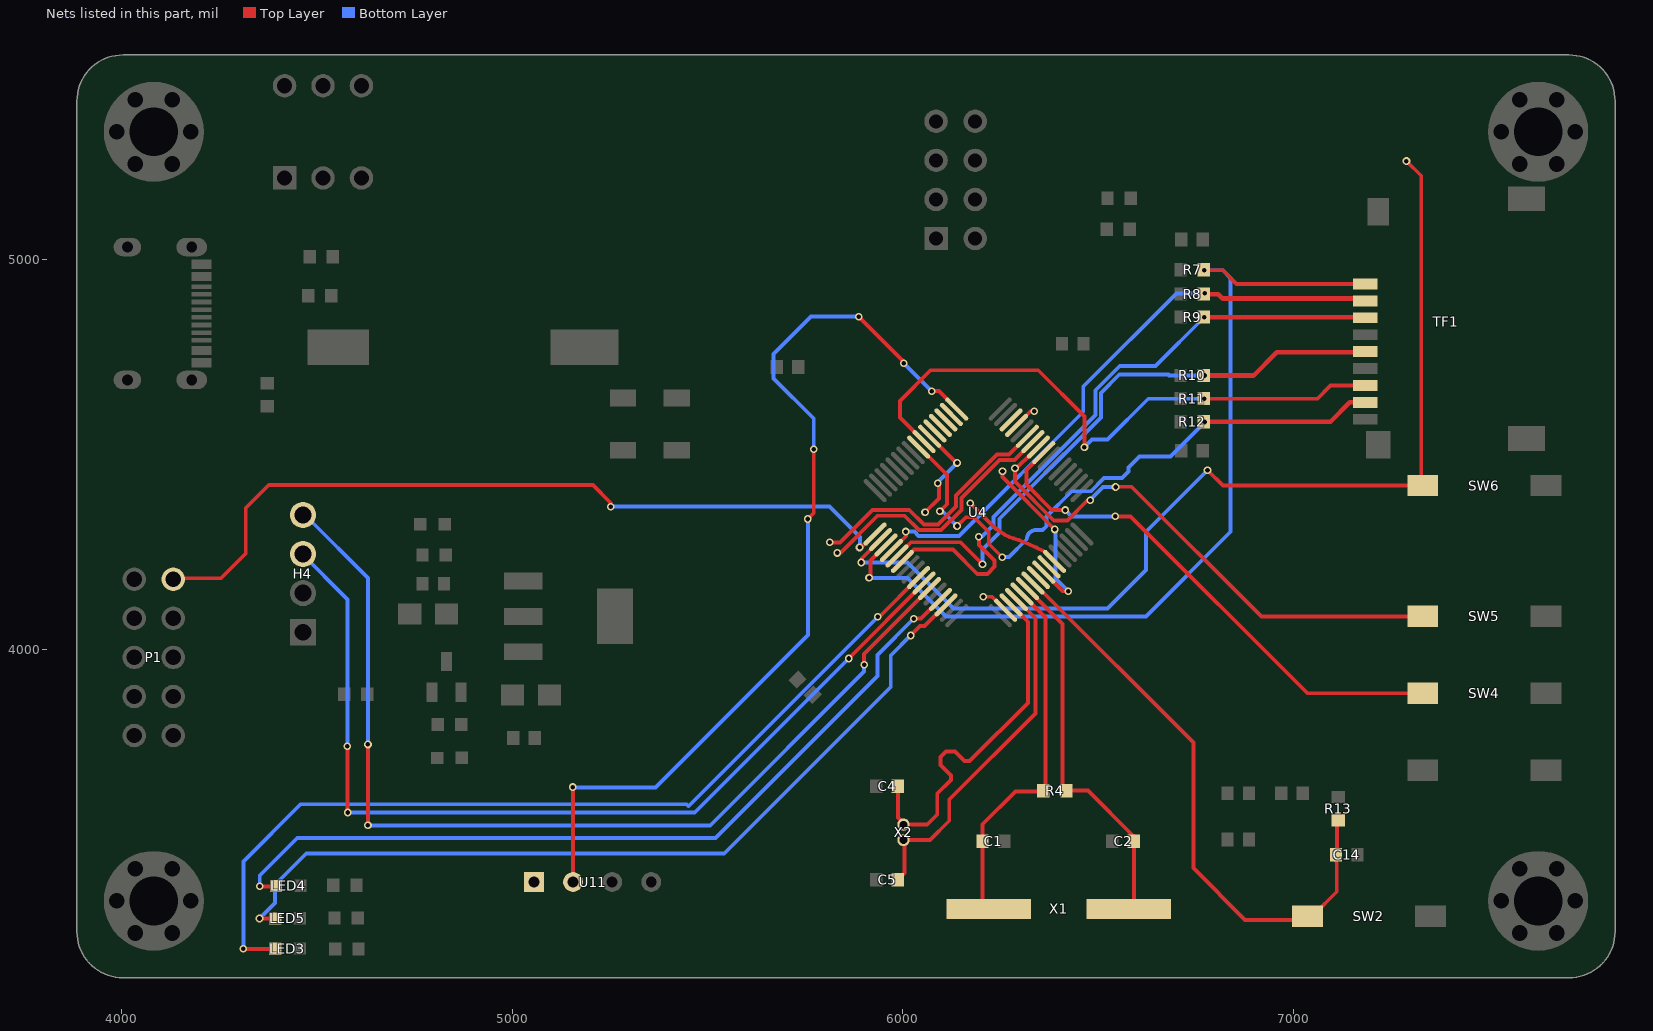
[diagram p0: the nets of this part, all layers, seen from the top]
# Altium PCB MISC52064.pcbdoc (part 2 of 2)
Units mil, origin at the board's own origin, x right, y up, seen from the top; angles counter-clockwise.
Board outline 3937.01 x 2362.2 mil, 2 copper layers (Top Layer, Bottom Layer), stack 62.205 mil thick; 65 components, 70 nets, 266 pads, 190 vias.

## Via types
v1: diameter 19.68, hole 11.8, Top Layer to Bottom Layer, 190 vias

## Nets (pads, with @x,y where several pads share a name; then routed paths per layer and width w, separated by ;. In a path a pad name is that pad's centre, name@x,y a point inside that pad or via, vN(x,y) a via of type N, cw(c..) or ccw(c..) an arc to the next point about the centre after c; other vN are vias at no path point) (continued)
PA14: P1.2 U4.49 | length 2063.8
  Top Layer w10: P1.2@4127.52,4174.39 P1.2@4136.38,4183.24 ; P1.2@4132.65,4183.24 P1.2@4136.38,4183.24 ; v1@5252.59,4366.08 5252.59,4376.32 5206.94,4421.96 4377.35,4421.96 4318.51,4363.12 4318.51,4246.24 4255.51,4183.24 P1.2@4136.38,4183.24 ; v1(5889.48,4262.14) 5893.35,4262.14 5917.12,4285.9 U4.49@5917.99,4285.9
  Bottom Layer w10: v1(5252.98,4366.56) 5812.97,4366.56 5890.24,4289.28 5890.24,4262.35 v1@5890.42,4262.17
PA15: SW6.1 U4.50 | length 2631.1
  Top Layer w10: v1(5894.12,4223.6) 5894.12,4233.11 U4.50@5943.3,4282.29 ; v1(6779.94,4459.82) 6819.31,4420.45 SW6.1@7326.99,4420.45 ; v1@7290,5250.46 7326.99,5213.48 SW6.1@7326.99,4420.45 ; SW6.1@7331.13,4420.45 SW6.1@7326.99,4420.45
  Bottom Layer w10: v1(5894.12,4223.6) 6012.23,4223.6 6130.34,4105.49 6524.04,4105.49 6622.46,4203.91 6622.46,4302.34 v1(6779.94,4459.82)
  other v1: 7289.17,5251
PB0: U4.26 | length 664.7
  Top Layer w10: v1@5842.02,4249.68 5935.67,4343.32 6004.73,4343.32 6041.71,4306.34 6098.35,4306.34 6150.4,4358.39 6150.4,4388.83 6247.51,4485.94 6286.11,4485.94 U4.26@6338.64,4538.47
  other v1: 5832.43,4248.14
PB1: U4.27 | length 624.9
  Top Layer w10: v1@5816.27,4275.1 5839.45,4275.1 5922.13,4357.79 6016.73,4357.79 6054.15,4320.36 6090.07,4320.36 6136.4,4366.69 6136.4,4394.63 6241.71,4499.94 6272.21,4499.94 U4.27@6292.33,4520.06
  other v1: 5812.96,4275.08
PB5: LED3.1 U4.57 | length 2339.1
  Top Layer w10: v1(4312.24,3234.81) 4393.16,3234.81 LED3.1@4393.71,3235.35 ; v1(5936.24,4084.81) 5940.68,4084.81 U4.57@6040.73,4184.86
  Bottom Layer w10: v1(4312.24,3234.81) 4312.24,3458.81 4458.24,3604.81 5446.24,3604.81 5451.24,3599.81 v1(5936.24,4084.81)
PB6: H4.3 U4.58 | length 2436.4
  Top Layer w10: v1@4578,3750.53 v1@4578.95,3749.57 ; v1(4578.39,3753.08) 4579.24,3752.22 v1(4579.24,3583.81) ; v1(5861.75,3978.03) U4.58@6054.65,4170.94
  Bottom Layer w10: H4.3@4457.84,4250.39 4578.92,4129.31 4578.92,3754.31 v1@4579.34,3753.89 ; v1(4579.24,3583.81) 5467.53,3583.81 v1(5861.75,3978.03)
PB7: H4.4 U4.59 | length 2571.2
  Top Layer w10: v1(4631.09,3550.81) v1(4631.09,3757.97) ; v1(5901.24,3961.81) 5901.24,3989.69 U4.59@6068.57,4157.02
  Bottom Layer w10: H4.4@4475.84,4339.51 4631.25,4184.1 v1@4631.25,3754.77 ; v1(4631.09,3550.81) 5507.24,3550.81 5901.24,3944.81 v1(5901.24,3961.81)
PB8: LED4.1 U4.61 | length 2136.3
  Top Layer w10: v1(4354.24,3394.81) 4394.9,3394.81 LED4.1@4395.77,3395.67 ; v1(6028.24,4079.81) 6047.04,4079.81 U4.61@6096.41,4129.18
  Bottom Layer w10: v1(4354.24,3394.81) 4354.24,3422.81 4450.24,3518.81 5521.24,3518.81 5935.24,3932.81 5935.24,3986.81 v1(6028.24,4079.81)
PB9: LED5.1 U4.62 | length 2204.3
  Top Layer w10: v1(4353.74,3312.31) 4354.11,3312.67 LED5.1@4393.77,3312.67 ; v1(6020.24,4036.81) 6044.24,4060.81 6055.88,4060.81 U4.62@6110.33,4115.26
  Bottom Layer w10: v1(4353.74,3312.31) 4393.24,3351.81 4393.24,3398.81 4473.24,3478.81 5543.24,3478.81 5969.24,3904.81 5969.24,3985.81 v1(6020.24,4036.81)
PB10: U4.29 | length 47.2
  Top Layer w10: U4.29@6300.4,4583.97 6327.04,4610.61 v1(6336.56,4610.61)
PB11: U4.30
PB12: U4.33 U11.2 | length 2384.2
  Top Layer w10: v1(5155.24,3648.81) 5156.24,3647.81 U11.2@5156.24,3405.81 ; v1(5757.24,4334.81) 5772.24,4349.81 v1(5772.24,4513.81) ; v1(5887.24,4852.81) 6002.24,4737.81 v1(6002.24,4733.81) ; v1(6073.96,4662.09) 6092.43,4662.09 U4.33@6138.17,4616.35
  Bottom Layer w10: v1(5155.24,3648.81) 5156.24,3647.81 5367.24,3647.81 5757.24,4037.81 v1(5757.24,4334.81) ; v1(5772.24,4513.81) 5772.24,4591.81 5669.24,4694.81 5669.24,4756.81 5765.24,4852.81 v1(5887.24,4852.81) ; v1(6002.24,4733.81) v1(6073.96,4662.09)
PB13: U4.34
PB14: U4.35
PB15: U4.36
PC0: U4.8
PC1: U4.9 | length 426.8
  Top Layer w10: v1@6255.06,4457.95 6255.06,4442.22 v1(6389.01,4308.27) ; U4.9@6381.78,4177.29 6408.83,4150.24 v1@6423.56,4150.24
  Bottom Layer w10: v1@6390.73,4305.14 6390.73,4182.97 v1(6423.56,4150.14)
  other v1: 6255.32,4457.36
PC2: U4.10
PC3: U4.11 | length 230.9
  Top Layer w10: v1(6172.4,4375.21) 6173.72,4375.21 6237.79,4311.14 ; 6238.98,4309.74 ccw(c6333.82,4428.03) 6297.26,4280.89 ; 6297.61,4280.54 cw(c6095.87,3734.98) U4.11@6364.69,4250.8
PC4: SW4.1 U4.24 | length 1336.7
  Top Layer w10: U4.24@6360.87,4505 6316.24,4460.37 6316.24,4422.81 6381.24,4357.81 v1(6416.24,4357.81) ; v1(6543.72,4341.71) 6583.09,4341.71 7035.85,3888.95 SW4.1@7331.13,3888.95
  Bottom Layer w10: v1(6416.24,4357.81) 6432.35,4341.71 v1(6543.72,4341.71)
PC5: SW5.1 U4.25 | length 1348.6
  Top Layer w10: U4.25@6329.14,4502.85 6291.44,4465.15 v1(6287.35,4465.15) 6287.14,4464.95 6287.14,4430.47 6386.57,4331.04 6421.22,4331.04 6473.2,4383.01 v1@6478.82,4383.01 ; v1@6544.41,4417.27 6544.69,4417.55 6585.99,4417.55 6917.74,4085.8 SW5.1@7331.13,4085.8
  Bottom Layer w10: v1@6480.26,4384.7 6512.5,4416.94 v1(6544.74,4416.94)
  other v1: 6479.61,4383.08
PC6: U4.37
PC7: U4.38 | length 234.5
  Top Layer w10: v1(6057.11,4352.2) 6092.56,4387.65 6092.56,4422.88 v1@6089.34,4426.1 ; U4.38@6087.32,4528.43 6137.34,4478.41 v1(6139.08,4478.41)
  Bottom Layer w10: v1(6089.79,4426.76) 6089.79,4429.12 v1(6139.08,4478.41)
PC8: R11.1 TF1.7 U4.39 | length 1546.4
  Top Layer w10: U4.39@6054.65,4532.83 5992.54,4594.95 5992.54,4636.98 6071.28,4715.72 6346.87,4715.72 6464.98,4597.61 v1(6464.98,4518.87) ; v1(6771.24,4642.81) 7061.36,4642.81 7095.27,4676.71 TF1.7@7183.43,4676.71
  Bottom Layer w10: v1(6464.98,4518.87) 6484.67,4538.56 6524.04,4538.56 6628.29,4642.81 v1(6771.24,4642.81)
PC9: R12.1 TF1.8 U4.40 | length 1550.3
  Top Layer w10: U4.40@6051.52,4509.63 6112.92,4448.23 6112.92,4372.67 v1@6097.24,4356.99 ; v1(6139.04,4316.97) 6161.44,4339.37 6182.51,4339.37 6220.17,4301.71 6220.17,4271.5 v1(6254.56,4237.11)
  Top Layer w11.8: R12.1@6770.23,4584.2 7094.83,4584.2 7144.03,4633.4 TF1.8@7183.43,4633.4
  Bottom Layer w10: v1(6095.15,4354.94) 6101.07,4354.94 v1(6139.04,4316.97) ; v1@6253.59,4238.1 6272.33,4238.1 6317.31,4283.08 cw(c6341.79,4282.44) 6342.4,4306.92 ; 6341.36,4306.98 6358.15,4306.98 6367.65,4316.48 6367.65,4341.19 6432.51,4406.06 6481.81,4406.06 6515.29,4439.54 6560.68,4439.54 6577.38,4456.23 6577.38,4466.7 6605.46,4494.78 6684.78,4494.78 v1(6773.2,4583.21)
PC10: R7.1 TF1.1 U4.51 | length 2311.5
  Top Layer w10: v1(5913.8,4184.23) 5917.65,4188.07 5917.65,4228.81 U4.51@5957.22,4268.38 ; R7.1@6770.23,4972.74 6771.34,4971.63 6819.31,4971.63 6854.39,4936.55 TF1.1@7183.43,4936.55
  Bottom Layer w10: v1(5913.8,4184.23) 6012.23,4184.23 6110.65,4085.8 6622.46,4085.8 6839,4302.34 6839,4951.94 6819.31,4971.63 v1(6771.24,4971.63)
PC11: R8.1 TF1.2 U4.52 | length 1518.6
  Top Layer w10: U4.52@5992.76,4275.64 6007.86,4290.74 v1(6007.86,4302.71)
  Top Layer w11.8: R8.1@6770.23,4910.63 6807.85,4910.63 6819.31,4899.16 7177.53,4899.16 TF1.2@7183.43,4893.25
  Bottom Layer w10: v1(6007.86,4302.71) 6029.58,4302.71 6040.79,4291.49 6144.2,4291.49 6462.08,4609.37 6462.08,4674.12 6700.23,4912.27 v1(6773.01,4912.27)
PC12: R10.1 TF1.5 U4.53 | length 1514.6
  Top Layer w10: U4.53@6007.34,4261.15 6021.62,4275.44 6148.2,4275.44 v1@6204.83,4218.81
  Top Layer w11.8: R10.1@6770.23,4702.31 6898.05,4702.31 6957.11,4761.36 7181.46,4761.36 TF1.5@7183.43,4763.33
  Bottom Layer w10: v1(6203.99,4219.44) 6203.99,4256.55 6203.88,4256.66 6247.63,4300.42 6247.63,4335.53 6507.02,4594.92 6507.02,4657.43 6554.19,4704.6 6679.65,4704.6 6681.96,4702.29 v1(6772.18,4702.29)
PC13: U4.2 | length 45.1
  Top Layer w10: v1(6205.96,4135.91) 6228.94,4135.91 U4.2@6244.55,4120.3
PC14: C4.2 U4.3 X2.1 | length 915.5
  Top Layer w10: C4.2@5987.32,3651.05 5987.32,3570.42 X2.1@6003.36,3554.39 ; X2.1@6001.74,3552.77 X2.1@6004.98,3552.77 ; X2.1@6005.27,3552.48 X2.1@6004.98,3552.77 ; U4.3@6297.08,4095.24 6320.46,4071.86 6320.46,3864.49 6171.33,3715.36 6158.22,3715.36 6133.91,3739.67 6110.47,3739.67 6096.6,3725.81 6096.6,3705.2 6123,3678.8 6123,3667.23 6088.37,3632.6 6088.37,3578.49 6062.65,3552.77 X2.1@6004.98,3552.77
PC15: C5.2 U4.4 X2.2 | length 922.6
  Top Layer w10: C5.2@5987.32,3411.66 6004.13,3428.48 X2.2@6004.13,3511.07 ; X2.2@6001.74,3513.4 X2.2@6006.55,3513.4 ; X2.2@6006.16,3513.01 X2.2@6006.55,3513.4 ; U4.4@6291.27,4129.18 6339.64,4080.82 6339.64,3837.42 6119.07,3616.84 6119.07,3562.68 6069.79,3513.4 X2.2@6006.55,3513.4
PD0: C1.2 R4.2 U4.5 X1.2 | length 939.2
  Top Layer w10: X1.2@6205.75,3332.46 6204.34,3333.87 C1.2@6204.34,3510.27 6204.34,3553.66 6288.56,3637.87 R4.2@6357.18,3637.87 ; U4.5@6305.19,4143.1 6365.77,4082.52 6365.77,3652.59 R4.2@6355.77,3642.59
PD1: C2.2 R4.1 U4.6 X1.1 | length 943.4
  Top Layer w10: U4.6@6334.89,4140.92 6409.17,4066.64 6409.17,3649.48 R4.1@6419.17,3639.48 6420.1,3640.4 6473.62,3640.4 C2.2@6589.96,3524.07 ; X1.1@6588.57,3337.57 6591.39,3340.38 C2.2@6591.39,3510.06 C2.2@6591.39,3524.07
PD2: R9.1 TF1.3 U4.54 | length 1670.2
  Top Layer w10: U4.54@5980.15,4208.04 6028.65,4256.54 6128.79,4256.54 6190.72,4194.61 6216.45,4194.61 6234.97,4213.12 6234.97,4228.5 6195.01,4268.45 v1@6195.01,4285.85
  Top Layer w11.8: R9.1@6770.23,4851.71 7181.66,4851.71 TF1.3@7183.43,4849.94
  Bottom Layer w10: v1@6194.86,4289.71 6202.39,4289.71 6232.57,4319.88 6232.57,4340.26 6493.02,4600.72 6493.02,4664.44 6555.48,4726.89 6647.29,4726.89 v1(6771.69,4851.3)
  other v1: 6194.42,4289.28
RESET: C14.2 R13.1 SW2.1 U4.7 | length 1440.5
  Top Layer w10: U4.7@6349.12,4157.64 6743.85,3762.91 6743.85,3441.25 6876.34,3308.77 SW2.1@7018.41,3308.77 ; SW2.1@7051.52,3322.4 7052.37,3322.4 7110.85,3380.88 7110.85,3458.2 C14.2@7109.31,3459.74 ; 7111.45,3493.61 R13.1@7111.45,3561.69
VCC: U11.1
pads on no net: P1.3 P1.9 SW1.1 SW1.4 SW1.5 SW1.6 TF1.9 U3.4 U6.2 U6.3 U6.6 U6.7 U11.3 USB1.1 USB1.2 USB1.3 USB1.4 USB1.A5 USB1.A8 USB1.B5 USB1.B8

## Polygon pours and split planes (outlines as drawn)
GND on Top Layer (solid, remove dead copper, pour order 2): 3712.18,5550.74 3712.18,3081.04 7994.47,3081.04 7994.47,5550.74
D+ on Top Layer (solid, remove dead copper, pour order 0): 4318.39,4870.68 4377.55,4870.68 4377.55,4779.4 4372.67,4774.53 4372.67,4779.76 4321.06,4831.37 4318.04,4831.37
GND on Bottom Layer (solid, remove dead copper, pour order 6): 3000,5646.93 3000,3000 7916.52,3000 7916.52,5646.93
5VOUT on Bottom Layer (solid, remove dead copper, pour order 4): 3787.66,3711.22 4284.49,3710.25 4283.63,3802.1 4346.9,3791.09 4426.63,3712.07 4868.15,3711.22 4878.86,3721.92 4960.59,3721.92 4968.88,3713.64 4968.88,3467.83 4930.81,3429.77 4735.49,3430.01 4734.63,3157.35 3787.66,3159.44

## Keep-outs
Top Layer:
  region: 4194.04,5050.95 4195.8,5052.71 4195.8,5004 4178.79,4986.99 4178.79,4938.21 4182.57,4934.43 4155.12,4906.98 4155.12,4790.3 4151.6,4786.78 4151.6,4785.9 4174.48,4763.01 4174.48,4669.71 4173.6,4668.83 4001.08,4668.83 3994.03,4675.87 3994.03,5035.01 4009.98,5050.95
  region: 6188.18,4715.09 6517.51,4385.77 6517.51,4321.19 6488.77,4292.46 6488.77,4264.37 6490.47,4262.67 6282.9,4055.1 6260.78,4055.1 6207.91,4107.97 6170.73,4107.97 5947.02,4331.68 5947.02,4374.28 5885.39,4435.91 6164.57,4715.09
Board Outline Layer:
  the board outline again, w10

## Other copper
Top Layer:
  region net PD2: 6032.19,4253 6025.12,4260.08 6018.46,4254.45 6026.82,4246.1
  region net PC11: 6004.32,4294.28 5990.63,4282.29 5998.98,4273.94 6010.99,4286.81
  region net GND: 5903.63,4453.36 5915.46,4440.97 5923.81,4449.32 5909.5,4461.64
  region net PA13: 5924.67,4475.31 5917.12,4468.73 5929.38,4454.88 5937.73,4463.23
  region net PA10: 6039.13,4443.43 6026.82,4457.67 6018.46,4449.32 6030.98,4437.43
  region net PA9: 5972.73,4524.94 5985.05,4510.56 5993.41,4518.91 5981.11,4530.7
  region net PC7: 6102.05,4506.63 6108.43,4514.39 6096.41,4527.26 6088.06,4518.91
  region net GND: 6238.01,4569.5 6243.95,4574.59 6235.6,4582.94 6230.93,4576.57
  region net PB10: 6330.58,4607.08 6323.51,4614.15 6310.76,4602.43 6319.11,4594.08
  region net BOOT1: 6336.56,4584.97 6329.49,4592.04 6326.4,4589.71 6334.21,4581.86
  region net PB0: 6293.01,4499.91 6300.04,4492.8 6313.54,4505 6305.19,4513.35
  region net 3.3V: 6398.46,4395.67 6410.98,4407.56 6402.63,4415.91 6390.32,4401.67
  region net GND: 6477.48,4461.54 6463.87,4449.32 6472.22,4440.97 6484.38,4454.29
  region net PA1: 6484.56,4247.94 6472.22,4262.81 6463.87,4254.45 6474.83,4243.52
  region net PA0: 6470.56,4235.12 6458.31,4248.89 6449.95,4240.54 6463.1,4228.43
  region net $1N7223: 6450.19,4214.31 6456.32,4222.33 6444.38,4234.97 6436.03,4226.61
  region net GND: 6442.56,4207.95 6430.47,4221.05 6422.12,4212.7 6435.92,4200.44
  region net PC1: 6401.01,4165.13 6388.71,4179.29 6380.35,4170.94 6392.99,4159
  region net PD1: 6359.22,4123.67 6346.95,4137.53 6338.6,4129.18 6351.63,4117.11
  region net PD0: 6345.22,4110.14 6333.03,4123.61 6324.68,4115.26 6338.15,4103.07
  region net PC15: 6324.23,4089.16 6331.3,4096.23 6319.11,4109.7 6310.76,4101.34
  region net PC14: 6317.45,4081.94 6305.19,4095.77 6296.84,4087.42 6309.91,4075.34
  region net PC13: 6225.4,4132.38 6235.6,4120.83 6243.95,4129.18 6232.48,4139.45
  region net $1N6590: 6282.78,4047.33 6289.45,4054.8 6277.35,4067.93 6269,4059.58
  region net PD1: 6596.39,3377.6 6586.39,3377.6 6573.89,3362.6 6608.89,3362.6
  region net PD0: 6209.34,3377.6 6199.34,3377.6 6186.84,3362.6 6221.84,3362.6
  region net 3.3V: 4949.95,4082.19 4979.95,4064.15 4979.95,4107.45 4949.95,4102.19
  region net 3.3V: 4431.36,4145.86 4421.91,4107.34 4429.28,4100.56 4468.31,4111.88
  region net 3.3V: 4488.06,4121.08 4507.07,4141.66 4507.07,4151.66 4485.81,4171.23
  region net 3.3V: 5450.4,4601.99 5476.35,4604.32 5455.14,4660.89 5388.21,4623.2
  region net $1N6590: 5427,4474.34 5439.5,4489.34 5404.5,4489.34 5417,4474.34
  region net $1N6590: 5358.21,4522.11 5358.21,4502.11 5388.21,4489.34 5388.21,4532.65
  region net $1N4980: 5242.08,4687.72 5229.2,4672.32 5250.42,4623.2 5250.42,4666.51
  region net $1N6590: 5347.35,4522.11 5317.35,4532.65 5317.35,4489.34 5347.35,4502.11
  region net $1N7223: 6881.24,3547.65 6870.5,3532.65 6901.99,3532.65 6891.24,3547.65
  region net 3.3V: 6414.69,4756.89 6423.39,4765.64 6392.19,4765.64 6404.69,4756.89
  region net 3.3V: 5804.61,3889.99 5777.11,3902.49 5774.33,3867.49 5801.83,3879.99
  region net 3.3V: 5742.58,4688.12 5748.34,4706.12 5716.85,4706.12 5730.58,4688.12
  region net GND: 5655.17,4695.51 5661.73,4706.12 5661.73,4741.55 5651.12,4705.6
  region net PC14: 5992.32,3618.33 6003.07,3633.33 5971.57,3633.33 5982.32,3618.33
  region net PC15: 6000.6,3432.01 5980.29,3429.38 6003.07,3402.66 6007.67,3424.94
  region net PD0: 6209.34,3477.56 6220.09,3492.56 6188.6,3492.56 6199.34,3477.56
  region net PD0: 6199.34,3542.99 6188.6,3527.99 6220.09,3527.99 6209.34,3542.99
  region net PD1: 6596.39,3477.34 6607.14,3492.34 6575.64,3492.34 6586.39,3477.34
  region net PD1: 6568.57,3538.38 6575.64,3513.64 6607.14,3527.78 6582.71,3538.38
  region net PD0: 6328.97,3642.87 6328.97,3632.87 6343.97,3622.47 6343.97,3655.37
  region net PD0: 6370.77,3671.49 6360.77,3671.49 6348.27,3656.49 6375.73,3656.49
  region net PD1: 6414.17,3671.49 6404.17,3671.49 6403.29,3656.49 6426.67,3656.49
  region net PD1: 6450.05,3635.4 6450.05,3645.4 6435.05,3656.49 6435.05,3622.9
  region net $1N7223: 6883.22,3665.76 6870.72,3650.76 6901.99,3650.76 6893.22,3665.76
  region net $1N7223: 6916.99,3628.05 6916.99,3638.05 6901.99,3650.55 6901.99,3615.55
  region net $1N7223: 6881.24,3600.33 6891.24,3600.33 6901.99,3615.33 6870.5,3615.33
  region net 3.3V: 7054.78,3628.05 7054.78,3638.05 7039.78,3650.05 7039.78,3616.04
  region net $1N7223: 6938.18,3628.05 6953.18,3616.04 6953.18,3650.05 6938.18,3638.05
  region net D-: 4246.28,4884.82 4246.28,4894.82 4231.28,4896.34 4231.28,4884.53
  region net D+: 4246.28,4875.68 4231.28,4876.65 4231.28,4864.84 4246.28,4865.68
  region net D+: 4246.28,4836.37 4231.28,4837.28 4231.28,4825.47 4246.28,4826.37
  region net 5VOUT: 4993.79,3726.71 5013.79,3726.71 5018.75,3756.71 4987.25,3756.71
  region net 5VOUT: 5011.64,3822.15 4991.64,3822.15 4987.25,3792.15 5018.75,3792.15
  region net 3.3V: 4840.14,4216.91 4820.14,4216.91 4810.1,4186.91 4841.6,4186.91
  region net 3.3V: 6705.91,4734.32 6695.04,4719.32 6726.79,4719.32 6715.91,4734.32
  region net 3.3V: 6705.91,4670.3 6715.91,4670.3 6726.79,4685.3 6695.04,4685.3
  region net PC12: 6803.81,4708.21 6786.11,4719.32 6786.11,4685.3 6803.81,4696.41
  region net 3.3V: 6705.91,4611.25 6715.91,4611.25 6726.79,4626.25 6695.04,4626.25
  region net 3.3V: 6705.91,4675.26 6695.04,4660.26 6726.79,4660.26 6715.91,4675.26
  region net 3.3V: 6680.04,4584.75 6680.04,4574.75 6695.04,4567.19 6695.04,4597.25
  region net 3.3V: 6705.91,4616.21 6695.04,4601.21 6726.79,4601.21 6715.91,4616.21
  region net PC9: 6803.81,4590.1 6786.11,4601.21 6786.11,4567.19 6803.81,4578.3
  region net 3.3V: 6705.91,4819.7 6715.91,4819.7 6726.79,4834.7 6695.04,4834.7
  region net PD2: 6803.81,4857.61 6786.11,4868.72 6786.11,4834.7 6803.81,4845.81
  region net 3.3V: 7146.6,3628.34 7131.6,3639.21 7131.6,3607.46 7146.6,3618.34
  region net 3.3V: 7082.58,3628.05 7097.58,3615.55 7097.58,3639.21 7082.58,3638.05
  region net $1N170341: 4873.81,3840.73 4863.81,3840.73 4853.64,3825.73 4885.39,3825.73
  region net $1N170394: 4812.27,3776.71 4824.77,3791.71 4794.32,3791.71 4802.27,3776.71
  region net $1N170394: 4812.27,3754.21 4802.27,3754.21 4792.8,3739.21 4824.29,3739.21
  region net $1N4980: 5229.68,4699.5 5254.68,4729.5 5184.68,4729.5 5209.68,4699.5
  region net PA14: 4154.77,4159.96 4184.49,4178.24 4183.64,4188.24 4150.96,4204.8
  region net PA13: 4155.33,4060.56 4184.6,4079.06 4183.48,4089.06 4150.3,4105.28
  region net 3.3V: 4062.48,3874.65 4075.1,3909.69 4069.03,3917.77 4035.43,3910.61
  region net PA9: 4155.85,3861.16 4184.71,3879.84 4183.31,3889.84 4149.64,3905.72
  region net PA10: 4146.24,3753.74 4182.42,3767.73 4185.18,3777.73 4158.21,3797.12
  region net 3.3V: 4840.14,4195.61 4846.02,4225.61 4814.27,4225.61 4820.14,4195.61
  region net 3.3V: 4876.02,4253.28 4846.02,4259.62 4846.02,4225.61 4876.02,4233.28
  region net $1N123092: 4760.82,4289.62 4754.95,4259.62 4786.7,4259.62 4780.82,4289.62
  region net BOOT1: 6593.9,5044.32 6597.17,5059.32 6571.4,5059.32 6583.9,5044.32
  region net 5VOUT: 4991.64,3941.17 4972.11,3911.17 5031.16,3911.17 5011.64,3941.17
  region net 5VOUT: 5011.64,3827.67 5031.16,3857.67 4972.11,3857.67 4991.64,3827.67
  region net 3.3V: 4827.74,4050.44 4837.74,4050.44 4850.24,4065.44 4815.24,4065.44
  region net 3.3V: 4892.1,4082.19 4892.1,4102.19 4862.1,4118.94 4862.1,4065.44
  region net 3.3V: 4822.58,4148.94 4803.05,4118.94 4862.1,4118.94 4842.58,4148.94
  region net BOOT0: 6497.46,5147.09 6497.46,5132.95 6521.37,5139.17 6508.07,5173.19
  region net PA0: 7276.76,3700.6 7276.76,3690.6 7291.76,3678.1 7291.76,3713.1
  region net 3.3V: 7601.24,3654.33 7615.38,3654.33 7643.67,3664.93 7606.72,3677.48
  region net PC5: 7276.76,4090.8 7276.76,4080.8 7291.76,4068.3 7291.76,4103.3
  region net PC11: 7134.23,4893.26 7151.93,4879.45 7151.93,4907.05 7134.23,4905.06
  region net PD2: 7134.23,4857.61 7134.23,4845.81 7151.93,4836.14 7151.93,4863.74
  region net 3.3V: 7136.93,4801.63 7151.93,4792.83 7151.93,4820.43 7136.93,4811.63
  region net PC12: 7134.23,4767.26 7134.23,4755.46 7151.93,4749.53 7151.93,4777.13
  region net PC9: 7144.03,4639.3 7144.03,4627.5 7151.93,4619.6 7151.93,4647.2
  region net PC11: 6803.81,4904.73 6803.81,4916.53 6786.11,4927.64 6786.11,4893.62
  region net PC14: 6012.15,3540.96 6028.51,3547.77 6028.51,3557.77 6012.15,3564.58
  region net PC14: 6005,3568.18 5990.86,3573.96 5983.78,3566.89 5986.04,3554.08
  region net PC15: 5991.65,3501.31 5999.13,3485.91 6009.13,3487.45 6015,3504.9
  region net PC15: 6012.15,3501.59 6028.51,3508.4 6028.51,3518.4 6012.15,3525.21
  region net 5V: 4494.1,5187.53 4506.82,5156.64 4526.82,5157.07 4539.09,5188.5
  region net $1N175343: 4763.03,3892.52 4763.03,3880.52 4781.03,3866.95 4781.03,3907.52
  region net $1N170341: 4873.81,3851.95 4883.38,3866.95 4855.83,3866.95 4863.81,3851.95
  region net 3.3V: 4803.43,3994 4803.43,3984 4818.43,3971.5 4818.43,3994.9
  region net 3.3V: 4827.74,4009.9 4818.43,3994.9 4845.98,3994.9 4837.74,4009.9
  region net D+: 4451.7,4880.59 4478.36,4889.57 4462.31,4923.01 4451.7,4894.73
  region net D-: 4450.99,4996.96 4465.99,4988.89 4465.99,5019.46 4450.99,5006.96
  region net 3.3V: 4400.92,4597.79 4390.32,4626.08 4356.3,4607.41 4387.77,4596.8
  region net D+: 4367.67,4713.48 4356.3,4698.48 4390.17,4698.48 4377.67,4713.48
  region net $1N175343: 4663.5,3892.52 4645.5,3903.52 4645.5,3869.51 4663.5,3880.52
  region net PA9: 4536.43,3890.84 4536.43,3878.84 4554.43,3869.51 4554.43,3903.52
  region net PC13: 6212.47,4128.53 6222.7,4130.91 6222.7,4140.91 6212.47,4143.29
  region net 3.3V: 6402.3,4777.5 6404.69,4767.27 6414.69,4767.27 6417.07,4777.5
  region net 3.3V: 5729.2,4717.91 5730.58,4707.68 5742.58,4707.68 5743.96,4717.91
  region net PC11: 6000.48,4296.2 6002.86,4290.74 6012.86,4290.74 6015.24,4296.2
  region net PC5: 6296.56,4461.68 6303.59,4470.23 6298.69,4479.48 6289.64,4474.72
  region net PC5: 6279.83,4458.8 6282.14,4448.52 6292.14,4448.32 6294.59,4458.49
  region net PC9: 6104.98,4354.3 6110.53,4363.21 6103.48,4370.3 6094.56,4364.77
  region net 3.3V: 6696.2,4587.47 6686.23,4584.75 6687.43,4574.75 6697.95,4572.81
  region net 3.3V: 6395.34,4389.72 6401.34,4398.55 6395,4406.36 6386.03,4401.18
  region net PC7: 6066.94,4351.59 6072.48,4360.5 6065.41,4367.57 6056.5,4362.03
  region net PC7: 6138.46,4488.23 6129.48,4493.34 6123.31,4485.37 6129.41,4476.57
  region net PC7: 6084.54,4418.44 6087.56,4408.67 6097.56,4411.6 6098.71,4422.59
  region net BOOT1: 6596.29,4860.3 6593.9,4870.52 6583.9,4870.51 6581.52,4860.28
  region net BOOT1: 6368.11,4593.53 6356.59,4593.5 6351.42,4583.5 6361.33,4580.42
  region net BOOT0: 6591.19,4758.43 6582.29,4764.03 6575.12,4757.06 6580.61,4748.14
  region net BOOT0: 6133.99,4204.2 6128.76,4194.77 6140.7,4192.57 6148.51,4201.53
  region net PA0: 6553.09,4589.42 6562.01,4583.87 6569.08,4590.94 6563.53,4599.86
  region net PA1: 6532.51,4568.53 6541.42,4562.98 6548.49,4570.05 6542.95,4578.97
  region net PA1: 6549.62,4237.05 6539.37,4234.71 6539.23,4224.71 6549.43,4222.29
  region net PA1: 6610.6,4456.45 6601.69,4461.99 6594.62,4454.92 6600.16,4446.01
  region net PA0: 6527.88,4164.71 6535.72,4155.82 6547.57,4158.1 6542.38,4167.51
  region net PA0: 6528.9,4180.99 6519.49,4186.18 6517.21,4174.32 6526.11,4166.49
  region net PA0: 6654.73,4449.64 6645.81,4455.16 6638.79,4448.03 6644.37,4439.13
  region net PC12: 6778.71,4694.92 6788.93,4696.41 6788.91,4708.21 6778.68,4709.69
  region net PC9: 6780.42,4576.52 6790.51,4578.3 6789.32,4590.1 6778.93,4591.21
  region net PD2: 6778.5,4844.2 6788.67,4845.81 6788.17,4857.61 6777.89,4858.95
  region net PC11: 6778.2,4903.9 6788.7,4904.73 6790.7,4916.53 6780.65,4918.46
  region net PC5: 6551.69,4409.98 6561.77,4412.55 6561.15,4422.55 6550.78,4424.71
  region net PC5: 6471.15,4388.11 6463.05,4379.94 6466.49,4369.24 6475.68,4374.06
  region net PC3: 6172.72,4365.37 6181.68,4360.17 6188.08,4367.92 6182.12,4376.75
  region net 3.3V: 5860.23,4574.85 5862.61,4564.62 5872.61,4564.62 5874.99,4574.85
  region net $1N6590: 5374.26,4322.57 5379.74,4331.49 5372.55,4338.45 5363.65,4332.84
  region net $1N6590: 5473.94,4108.22 5482.85,4102.68 5489.92,4109.75 5484.38,4118.66
  region net PB0: 5840.08,4241.95 5849.13,4249.71 5847.09,4261.81 5837.62,4256.51
  region net PB0: 5840.08,4241.95 5849.13,4249.71 5847.09,4261.81 5837.62,4256.51
  region net PB1: 5819.49,4267.71 5829.7,4270.1 5829.68,4280.1 5819.45,4282.48
  region net PA14: 5260.05,4373.4 5252.69,4383.29 5239.18,4382.66 5245.3,4372.71
  region net PA14: 5260.05,4373.4 5252.69,4383.29 5239.18,4382.66 5245.3,4372.71
  region net PA14: 5898.74,4258.81 5905.68,4267.4 5900.66,4276.52 5891.62,4271.74
  region net PA13: 5293.95,4394.79 5296.39,4384.61 5306.39,4384.79 5308.71,4395.06
  region net PA13: 5718.12,4413.74 5715.74,4423.96 5705.74,4423.96 5703.36,4413.74
  region net PA9: 5967.35,4535.64 5969.74,4530 5979.74,4530 5982.12,4535.64
  region net PA10: 6042.86,4442.3 6034.08,4448.48 6026.01,4442.4 6031.07,4433.42
  region net PA9: 5824.44,4715.77 5814.22,4713.39 5814.22,4703.39 5824.44,4701
  region net PA10: 5831.83,4682.43 5821.61,4680.05 5821.61,4670.05 5831.83,4667.67
  region net PA9: 5692.09,4548.91 5689.45,4558.94 5679.45,4558.09 5677.38,4547.65
  region net PA9: 4376.23,3892.22 4366.01,3889.84 4366.01,3879.84 4376.23,3877.46
  region net PA9: 4389.25,3877.46 4399.47,3878.84 4399.47,3890.84 4389.25,3892.22
  region net PA10: 5681.2,4489.85 5686.71,4498.77 5679.58,4505.78 5670.67,4500.2
  region net PA10: 4418.72,3780.11 4408.5,3777.73 4408.5,3767.73 4418.72,3765.34
  region net PC12: 6204.76,4229.25 6195.85,4234.86 6188.68,4227.89 6194.16,4218.97
  region net PD2: 6187.44,4282.34 6190.01,4272.25 6200.01,4272.86 6202.18,4283.23
  region net PA15: 7288.76,5241.17 7297.69,5235.71 7304.61,5242.93 7298.97,5251.83
  region net PB10: 6329.81,4617.77 6319.82,4610.46 6320.27,4596.77 6330.29,4603.02
  region net PB10: 6329.81,4617.77 6319.82,4610.46 6320.27,4596.77 6330.29,4603.02
  region net PC9: 6148.86,4316.35 6154.4,4325.26 6147.33,4332.34 6138.42,4326.79
  region net PC9: 6255.17,4246.94 6246.26,4252.48 6239.19,4245.41 6244.73,4236.5
  region net PC1: 6417.13,4157.58 6408.83,4155.24 6408.83,4145.24 6416.98,4142.82
  region net PC1: 6247.77,4451.04 6250.06,4442.22 6260.06,4442.22 6262.53,4450.66
  region net GND: 6740.97,3853.9 6738.59,3864.12 6728.59,3864.12 6726.21,3853.9
  region net GND: 6193.84,4648.84 6201.8,4644.14 6208.88,4651.21 6204.53,4659.03
  region net GND: 5544.38,4677.38 5554.59,4679.78 5554.55,4689.78 5544.32,4692.14
  region net GND: 6497.51,4479.6 6488,4472.05 6489.3,4459.21 6498.99,4464.91
  region net GND: 6497.51,4479.6 6488,4472.05 6489.3,4459.21 6498.99,4464.91
Bottom Layer:
  region net PB6: 4461.49,4211.87 4500.5,4200.66 4507.83,4207.47 4498.27,4246.02
  region net PB7: 4466.53,4311.74 4504.55,4303.73 4510.82,4311.6 4497.77,4351.03
  region net 3.3V: 5732.19,4715.61 5740.54,4707.97 5750.6,4712.05 5745.87,4721.16
  region net PC11: 6014.37,4295.32 6024.59,4297.71 6024.59,4307.71 6014.37,4310.09
  region net PC9: 6098.77,4345.79 6107.91,4341.02 6111.67,4351.41 6103.79,4359.67
  region net 3.3V: 6697.02,4588.29 6686.8,4585.9 6686.82,4575.9 6697.04,4573.53
  region net 3.3V: 6257.27,4626.68 6256.84,4637.27 6244.84,4640.06 6242.89,4630.02
  region net 3.3V: 6395.47,4391.08 6400.88,4400.01 6393.56,4406.84 6384.67,4401.15
  region net PC7: 6129.26,4479.03 6123.72,4470.12 6130.79,4463.04 6139.7,4468.59
  region net PC7: 6099.58,4427.82 6104.56,4436.82 6096.27,4442.67 6087.52,4436.34
  region net BOOT1: 6579.14,4854.91 6573.37,4846.04 6580.07,4838.6 6589.01,4843.94
  region net BOOT1: 6378.25,4590.06 6376.07,4600.42 6366.07,4601 6363.51,4590.9
  region net BOOT0: 6583.93,4756 6573.71,4753.62 6573.71,4743.62 6583.93,4741.24
  region net BOOT0: 6152.12,4207.56 6158.16,4216.38 6151.88,4224.24 6142.91,4219.1
  region net PA0: 6588.89,4667.61 6591.27,4657.39 6601.27,4657.39 6603.65,4667.61
  region net PA1: 6553.83,4671.85 6556.22,4661.63 6566.22,4661.63 6568.6,4671.85
  region net PA0: 6560.92,4605.94 6558.46,4609.1 6548.46,4609.1 6546.16,4605.56
  region net PA1: 6538.44,4586.64 6535.42,4596.41 6525.42,4593.55 6524.24,4582.58
  region net PA1: 6565.86,4228.97 6571.4,4237.88 6564.33,4244.95 6555.42,4239.4
  region net PA1: 6603.47,4454.01 6593.94,4451.62 6593.94,4441.62 6603.47,4439.24
  region net PA0: 6543.72,4171.96 6549.24,4180.88 6542.12,4187.9 6533.21,4182.32
  region net PA0: 6644.37,4440.48 6638.8,4431.57 6645.84,4424.46 6654.76,4429.99
  region net PC12: 6765.67,4709.67 6755.45,4707.29 6755.45,4697.29 6765.67,4694.91
  region net PC9: 6763.38,4583.82 6757.83,4574.91 6764.9,4567.84 6773.81,4573.38
  region net PD2: 6761.87,4851.92 6756.32,4843 6763.39,4835.93 6772.31,4841.48
  region net PC11: 6766.5,4919.65 6756.27,4917.27 6756.27,4907.27 6766.5,4904.88
  region net PC5: 6538.23,4424.32 6528,4421.94 6528,4411.94 6538.23,4409.56
  region net 3.3V: 5872.82,4589.71 5864.7,4597.95 5853.81,4594.7 5858.68,4585.48
  region net $1N6590: 5357.04,4316.52 5359.43,4306.29 5369.43,4306.29 5371.81,4316.52
  region net $1N6590: 5475.93,4127.79 5467.08,4133.67 5459.46,4127.15 5464.72,4118.19
  region net PA14: 5259.49,4359.17 5269.71,4361.56 5269.71,4371.56 5259.49,4373.94
  region net PA14: 5897.34,4268.05 5895.24,4278.47 5885.24,4279.25 5882.63,4269.2
  region net PA13: 5309.99,4396.98 5319.76,4400.08 5315.78,4410.08 5304.53,4410.7
  region net PA13: 5702.77,4413.01 5692.95,4410.08 5695.19,4400.08 5706,4398.6
  region net PA9: 5975.35,4551.97 5966.44,4557.51 5959.37,4550.44 5964.91,4541.53
  region net PA10: 6041.5,4442.48 6032.59,4448.03 6025.52,4440.96 6031.06,4432.04
  region net PA9: 5837.79,4701.31 5847.91,4703.83 5847.45,4713.83 5837.12,4716.05
  region net PA10: 5843.88,4666.91 5854.42,4668.82 5854.96,4678.82 5845.73,4681.56
  region net PA9: 5675.47,4542.41 5669.93,4533.5 5677,4526.43 5685.91,4531.97
  region net PA9: 4382.87,3894.68 4373.93,3900.04 4367.21,3892.62 4372.96,3883.74
  region net PA10: 5661.55,4491 5656.01,4482.09 5663.08,4475.01 5671.99,4480.56
  region net PA10: 4432.37,3779.51 4429.87,3789.64 4419.87,3789.27 4417.61,3778.96
  region net PC12: 6211.37,4225.95 6208.99,4236.17 6198.99,4236.17 6196.61,4225.95
  region net PD2: 6202.33,4283.44 6211.09,4291.33 6208.59,4302.97 6199.23,4297.87
  region net PB6: 4586.11,3759.18 4583.92,3769.53 4573.92,3770.08 4571.37,3759.98
  region net PB7: 4638.58,3764.36 4636.25,3774.62 4626.25,3774.79 4623.82,3764.61
  region net PC9: 6139.65,4326.79 6130.74,4332.34 6123.67,4325.26 6129.21,4316.35
  region net PC9: 6261.78,4230.42 6271.78,4233.1 6270.77,4243.1 6260.29,4245.11
  region net PC1: 6424.18,4159.96 6415.27,4165.5 6408.2,4158.43 6413.74,4149.52
  region net PC1: 6382.88,4300.57 6385.73,4290.69 6395.73,4292.47 6397.42,4303.16
  region net GND: 6194.08,4648.83 6202.99,4643.28 6210.06,4650.35 6204.52,4659.27
  region net GND: 6445.22,4784.91 6439.67,4776 6446.74,4768.93 6455.66,4774.47
  region net GND: 6511.24,4465.53 6521.46,4467.91 6521.46,4477.91 6511.24,4480.29
  region net GND: 6638.51,4537.53 6628.12,4535.39 6627.46,4525.39 6637.53,4522.8

## Silkscreen, mask and mechanical layers (free items; w line width, h text height)
Top Silkscreen Layer:
  circle w12: c4079.59,3359.15 r163.88
Bottom Silkscreen Layer:
  region: 4191.74,4181.55 cw(c4133.76,4181.55) 4075.77,4181.55 cw(c4133.76,4181.55)
  lines w10: 4200.69,4192.26 4286.08,4192.26 4286.47,4191.87 ; 4265.99,4170.6 4355.92,4172.09 ; 4279.62,4589.35 4364.86,4588.29 ; 4333.01,4193.41 4333.4,4193.03 4382.24,4193.03 ; 4369.12,4410.06 4369.12,4559.78 ; 4372.58,4252.84 4372.58,4342.84 ; 4391.91,4588.68 4393.06,4587.52 4393.06,4490.02 ; 4393.06,4183.03 4394.79,4184.76 4394.79,4273.61 ; 4393.35,4337.22 4393.35,4451.46
  lines w12: 3999.77,4310.4 4208.7,4310.4 ; 3999.77,4391.47 4208.7,4391.47 ; 3999.77,4470.53 4208.7,4470.53 ; 4003.02,4547.18 4208.59,4547.18 ; 6549.09,5125.13 6656.43,5125.13 ; 3940.71,4240.88 3940.71,4621.43 4267.76,4621.43 4267.76,4240.88 3940.71,4240.88 ; 6548.49,4976.15 6548.49,5267.44 6656.48,5267.44 6656.48,4976.15 6548.49,4976.15
  text "B0" at 6647.13,5247.82 h78.74 r90
  text "B1" at 6643.54,5088.65 h78.74 r90
  text "SCK" at 4254.69,4541.17 h78.74
  text "RST" at 4083.09,4538.56 h78.74
  text "NC" at 4077.79,4470.78 h78.74
  text "SWD" at 4252.73,4466.19 h78.74
  text "GND" at 4181.52,4381.08 h78.74
  text "TX" at 4245.24,4308.11 h78.74
  text "3.3" at 4111.89,4305.61 h78.74
  text "NC" at 4084.42,4233.69 h78.74
  text "RX" at 4237.76,4231.73 h78.74
Top Paste Mask Layer:
  region: 5726.69,3561.39 5726.69,3506.22 5886.04,3506.22 5886.04,3561.39
Top Solder Mask Layer:
  region: 5723.37,3565.38 5723.37,3502.74 5889.43,3502.74 5889.43,3565.38